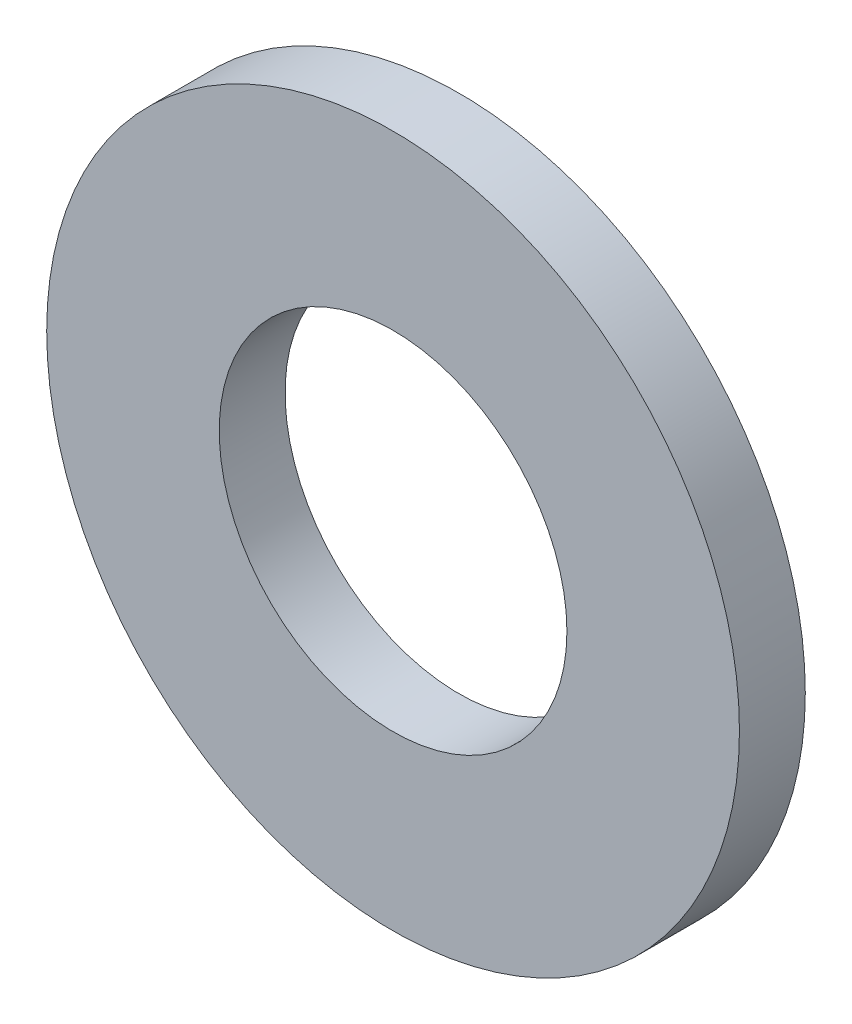
from build123d import *

# Parameters (mm, degrees)
SKETCH1_R           = 13.15
SKETCH1_R_2         = 6.6
BOSS_EXTRUDE1_DEPTH = 1.25


with BuildPart() as part:
    # Sketch1 → Boss-Extrude1 (new, symmetric)
    with BuildSketch(Plane.XY):
        Circle(SKETCH1_R)
        Circle(SKETCH1_R_2, mode=Mode.SUBTRACT)
    extrude(amount=BOSS_EXTRUDE1_DEPTH, both=True)


solid = part.part
